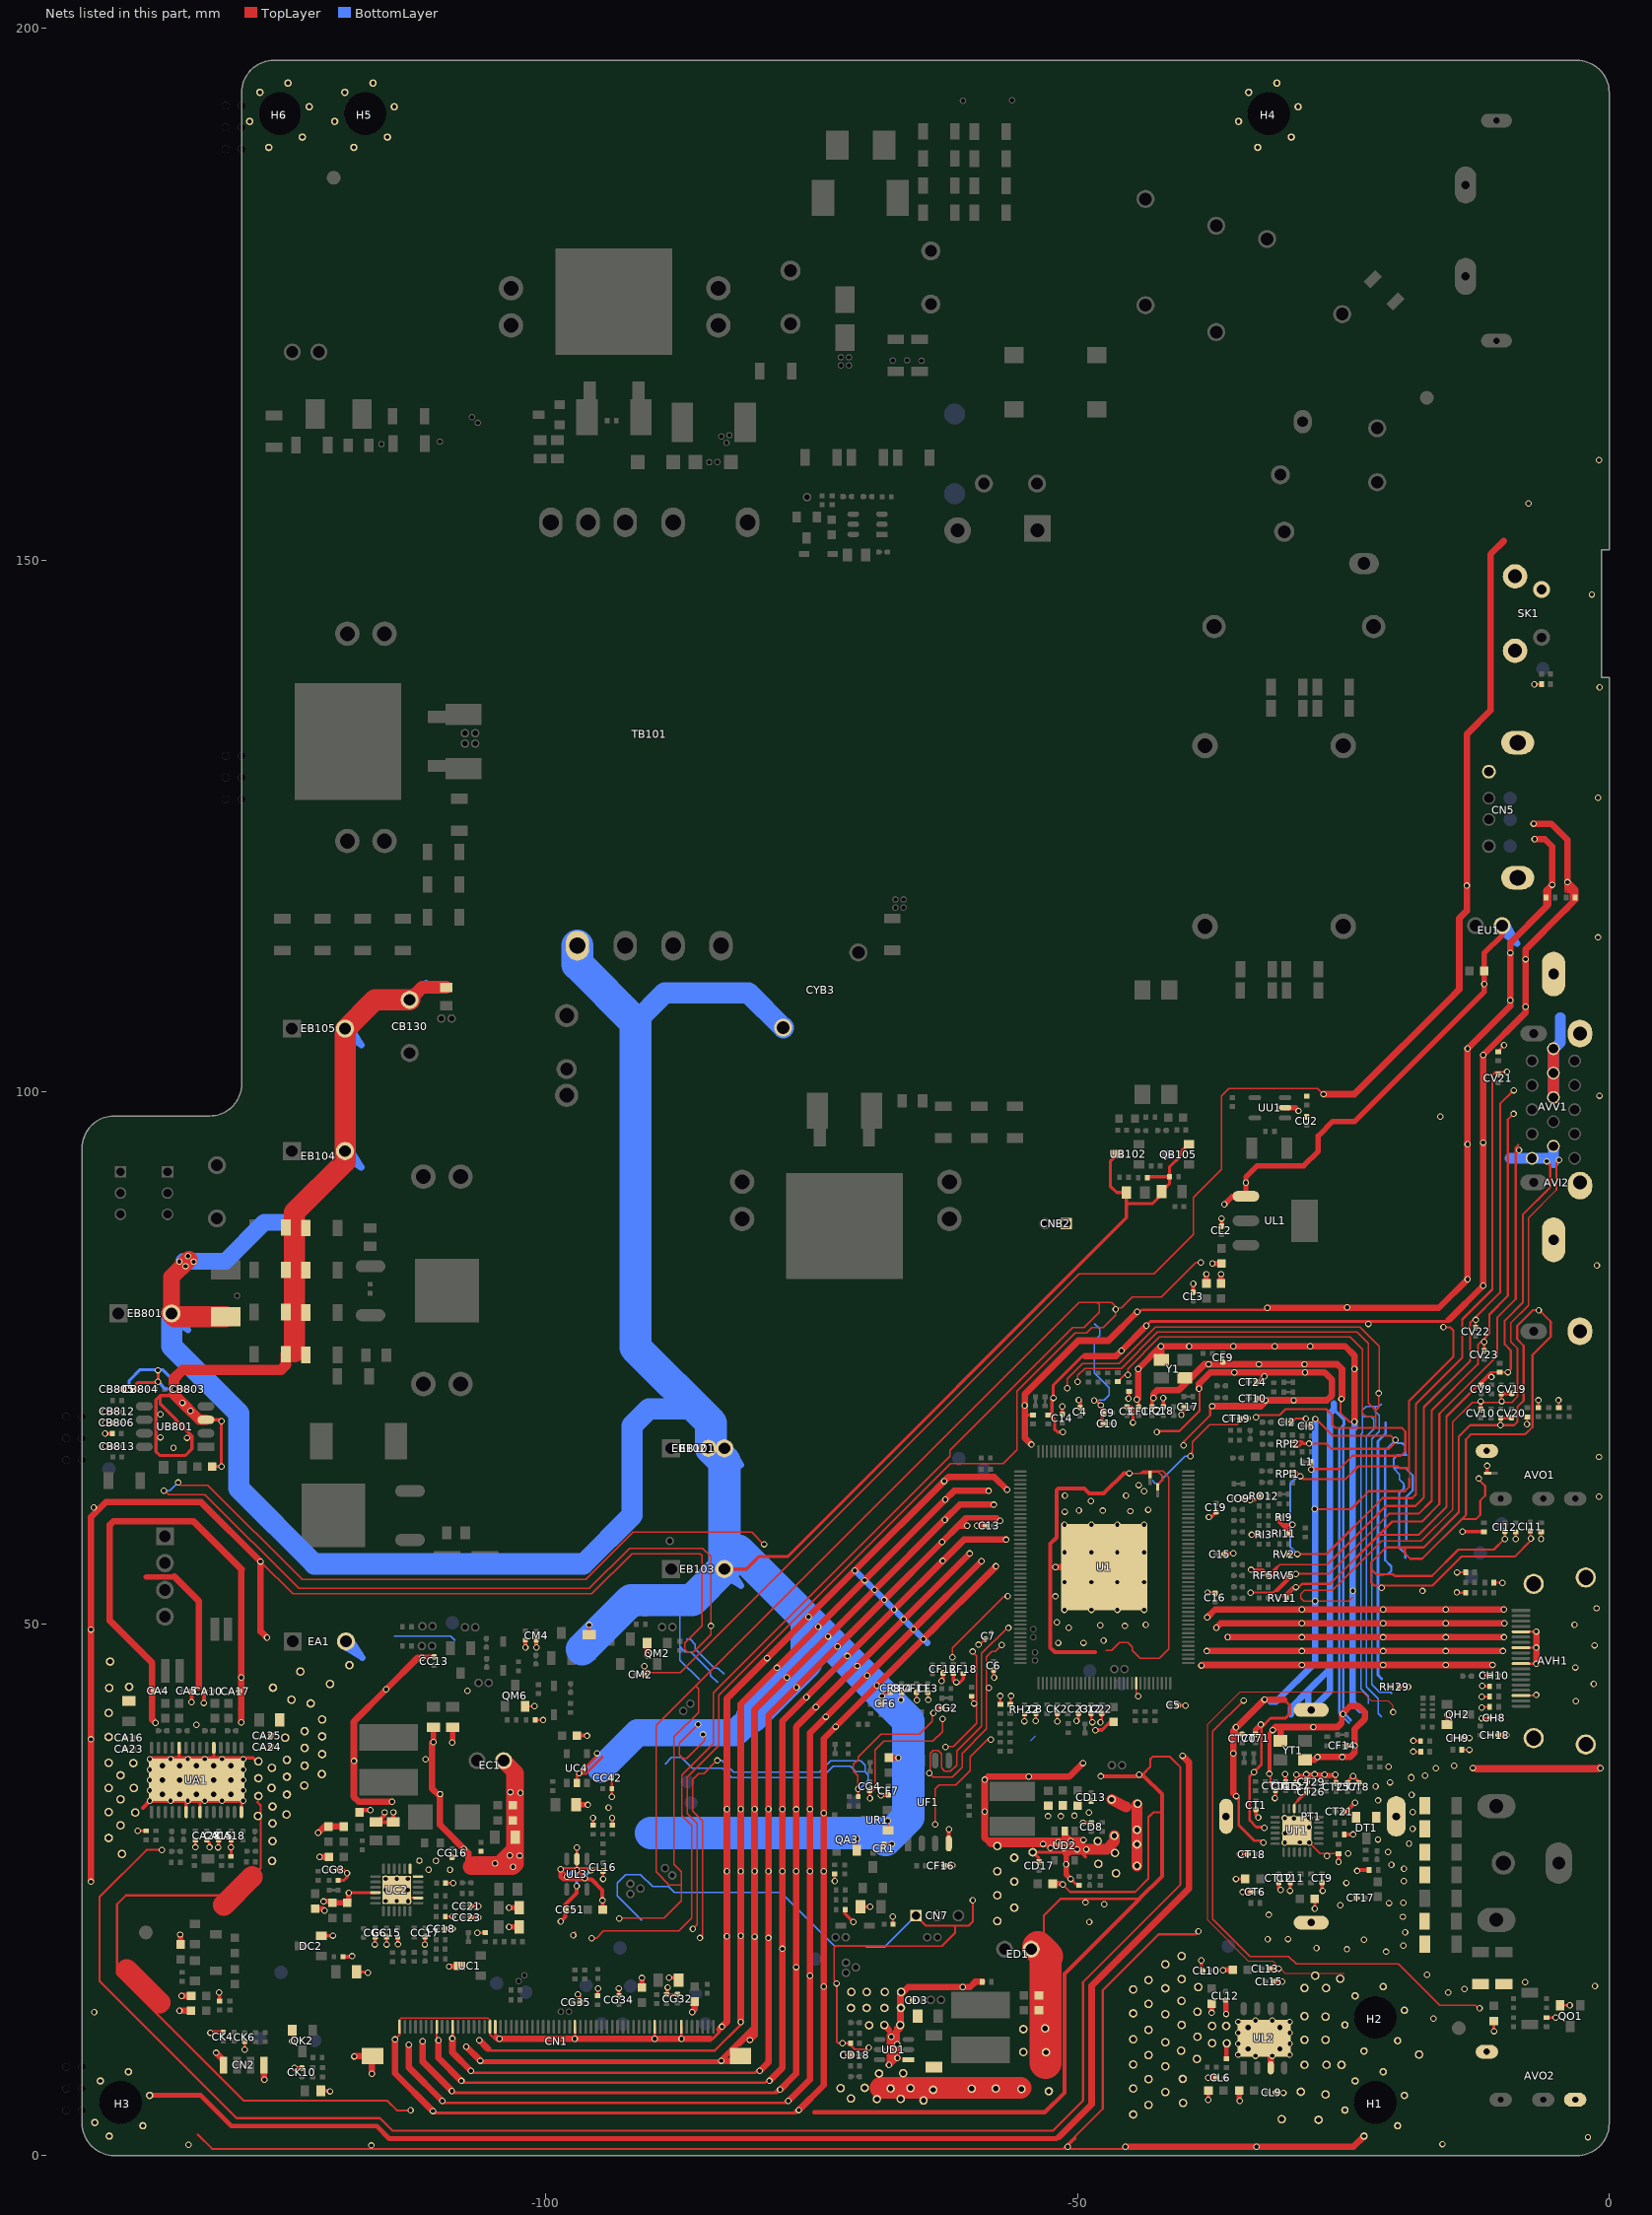
[diagram p0: the nets of this part, all layers, seen from the top]
# Altium PCB MISC86383-9.PcbDoc (part 9 of 18)
Units mm, origin at the board's own origin, x right, y up, seen from the top; angles counter-clockwise.
Board outline 143.6 x 197 mm, 2 copper layers (TopLayer, BottomLayer), stack 1.571 mm thick; 743 components, 401 nets, 2996 pads, 1077 vias.
Unrouted connection lines stored in the file: 4.

## Via types
v1: diameter 0.6, hole 0.4, TopLayer to BottomLayer, tented both sides, 993 vias
v2: diameter 0.6, hole 0.4, TopLayer to BottomLayer, 65 vias
v3: diameter 0.7, hole 0.5, TopLayer to BottomLayer, tented both sides, 15 vias
v4: diameter 0.8, hole 0.5, TopLayer to BottomLayer, tented both sides, 4 vias

## Nets (pads, with @x,y where several pads share a name; then routed paths per layer and width w, separated by ;. In a path a pad name is that pad's centre, name@x,y a point inside that pad or via, vN(x,y) a via of type N, cw(c..) or ccw(c..) an arc to the next point about the centre after c; other vN are vias at no path point) (continued)
GND: AVH1.5 AVH1.8 AVH1.11 AVH1.17 AVH1.20 AVH1.21 AVH1.22 AVH1.23 AVI2.2 AVI2.4 AVI2.6 AVO1.1 AVO2.1 AVO2.3 AVV1.5 AVV1.6 AVV1.7 AVV1.8 AVV1.10 AVV1.16 AVV1.17 C3.1 C4.1 C5.1 C6.1 C7.1 C8.1 C9.1 C10.1 C11.1 C12.1 C13.1 C14.1 C15.1 C16.1 C17.1 C18.1 C19.1 C22.1 C23.1 CA4.2@-136.92,43.698 CA4.2@-136.745,43.698 CA5.2@-133.314,43.673 CA5.2@-133.489,43.673 CA10.2@-131.982,43.66 CA10.2@-132.157,43.66 CA15.2@-130.762,29.658 CA15.2@-130.762,29.833 CA16.1 CA17.1 CA18.2@-129.594,29.658 CA18.2@-129.594,29.833 CA23.1 CA24.1 CA25.1 CA28.1 CA31.1 CA32.1 CA36.1 CB115.2 CB130.1 CB801.1 CB803.2@-133.987,72.074 CB803.2@-134.162,72.074 CB804.2@-138.5,72.06 CB804.2@-138.325,72.06 CB805.1 CB806.2@-140.77,68.885 CB806.2@-140.595,68.885 CB812.1 CB813.1 CC1.1 CC2.1 CC4.2 CC5.2 CC7.1 CC8.1 CC9.2 CC10.2 CC11.2 CC12.1 CC13.1 CC15.2@-114.98,20.53 CC15.2@-114.98,20.705 CC17.1 CC18.1 CC19.2 CC20.2 CC21.2@-107.018,23.463 CC21.2@-107.193,23.463 CC23.1 CC29.2 CC30.2 CC33.1 CC34.1 CC38.1 CC42.2@-93.783,35.496 CC42.2@-93.958,35.496 CC43.1 CC50.2 CC51.1 CD1.1 CD2.2 CD3.1 CD7.1 CD8.1 CD9.1 CD10.1 CD13.1 CD14.1 CD15.1 CD16.1 CD17.1 CD18.1 CF1.1 CF2.1 CF3.2@-64.069,43.521 CF3.2@-64.069,43.696 CF4.2@-66.548,43.517 CF4.2@-66.548,43.692 CF6.2@-68.297,42.469 CF6.2@-68.472,42.469 CF7.2@-67.783,33.871 CF7.2@-67.783,34.046 CF8.2@-67.615,43.517 CF8.2@-67.615,43.692 CF9.1 CF10.1 CF11.2@-65.151,43.517 CF11.2@-65.151,43.692 CF12.2@-62.649,45.32 CF12.2@-62.649,45.495 CF14.1 CF16.2@-62.458,27.254 CF16.2@-62.633,27.254 CG2.2@-62.582,42.05 CG2.2@-62.757,42.05 CG3.2@-119.532,26.878 CG3.2@-119.707,26.878 CG4.2@-69.545,34.297 CG4.2@-69.545,34.472 CG6.2@-116.046,20.53 CG6.2@-116.046,20.705 CG14.2 CG16.1 CG22.2 CG28.2 CG31.1 CG32.1 CG33.1 CG34.1 CG35.2@-96.743,14.402 CG35.2@-96.918,14.402 CH8.1 CH9.1 CH10.1 CH18.1 CI2.1 CI5.1 CI11.2@-7.417,58.706 CI11.2@-7.417,58.881 CI12.2@-9.804,58.83 CI12.2@-9.804,58.655 CK2.2@-51.903,41.553 CK2.2@-51.903,41.728 CK4.2@-130.333,11.424 CK4.2@-130.333,11.599 CK6.1 CK10.1 CL1.1 CL2.1 CL3.1 CL4.1 CL5.1 CL6.1 CL7.1 CL8.1 CL9.1 CL10.1 CL11.2 CL12.1 CL13.2@-31.884,17.577 CL13.2@-32.059,17.577 CL14.2 CL15.2@-31.528,16.358 CL15.2@-31.703,16.358 CL16.2@-94.615,26.689 CL16.2@-94.615,26.864 CM2.2@-90.697,45.212 CM2.2@-90.872,45.212 CM4.2@-100.902,48.444 CM4.2@-100.902,48.619 CM5.1 CN1.1 CN1.8 CN1.11 CN1.18 CN1.19 CN1.34 CN1.49 CN1.54 CN1.61 CN1.62 CN2.1 CN2.4 CN5.4 CN5.5 CN5.6 CN7.1 CNB2.1 CO9.1 CO77.2 CR1.1 CT1.1 CT2.1 CT5.1 CT6.2@-33.539,24.767 CT6.2@-33.714,24.767 CT7.1 CT8.1 CT9.2@-26.997,25.637 CT9.2@-26.997,25.812 CT10.2@-33.096,71.184 CT10.2@-33.271,71.184 CT11.1 CT12.2@-31.067,25.637 CT12.2@-31.067,25.812 CT14.1 CT15.1 CT17.2@-23.624,24.216 CT17.2@-23.799,24.216 CT18.1 CT19.1 CT21.2@-24.947,32.348 CT21.2@-25.122,32.348 CT24.1 CT25.2@-25.677,34.898 CT25.2@-25.677,35.073 CT26.1 CT27.2@-29.436,34.948 CT27.2@-29.436,35.123 CT29.1 CT41.1 CT42.1 CT43.1 CT44.1 CT45.1 CT46.1 CT47.1 CT48.1 CT70.2@-34.52,39.454 CT70.2@-34.52,39.629 CT71.1 CU1.1 CU2.2@-28.448,97.536 CU2.2@-28.448,97.711 CV9.1 CV10.1 CV19.1 CV20.1 CV21.1 CV22.1 CV23.1 CYB3.2 DB804.K DC2.3 DH2.A DH3.A DH6.A DH7.A DI1.A DI2.A DI3.A DI5.A DK1.A DK2.A DK6.A DK20.K DO1.A DO2.A DO3.A DR1.A DT1.1 DT1.3 DT2.A DT3.A DU1.A DU2.A DU3.A DU4.A DV1.A DV2.A DV3.A DV4.A DV5.A DV6.A DV7.A DV8.A EA1.2 EB101.2 EB102.2 EB103.2 EB104.2 EB105.2 EB801.2 EC1.2 ED1.2 EU1.2 H1.1 H1.2 H1.3 H1.4 H1.5 H1.6 H2.1 H2.2 H2.3 H2.4 H2.5 H2.6 H3.1 H3.2 H3.3 H3.4 H3.5 H3.6 H4.1 H4.2 H4.3 H4.4 H4.5 H4.6 H5.1 H5.2 H5.3 H5.4 H5.5 H5.6 H6.1 H6.2 H6.3 H6.4 H6.5 H6.6 L1.1 LT6.2 LT8.2 LT11.2 pad.VIA5@-17.882,9.5 pad.VIA5@-25.171,8.522 pad.VIA5@-25.298,16.612 pad.VIA5@-26.67,5.74 pad.VIA5@-26.67,10.871 pad.VIA5@-26.67,13.056 pad.VIA5@-26.568,8.534 pad.VIA5@-26.619,15.748 pad.VIA5@-27.33,3.353 pad.VIA5@-27.635,16.916 pad.VIA5@-28.651,8.534 pad.VIA5@-28.651,10.871 pad.VIA5@-28.651,13.106 pad.VIA5@-28.651,15.748 pad.VIA5@-29,5.994 pad.VIA5@-30.785,3.404 pad.VIA5@-35.966,10.54 pad.VIA5@-36.017,12.192 pad.VIA5@-37.338,10.566 pad.VIA5@-37.338,12.192 pad.VIA5@-38.71,11.176 pad.VIA5@-38.71,13.513 pad.VIA5@-38.645,15.833 pad.VIA5@-38.766,9.081 pad.VIA5@-40.073,4.944 pad.VIA5@-40.098,7.201 pad.VIA5@-40.195,16.592 pad.VIA5@-40.203,12.284 pad.VIA5@-40.208,18.748 pad.VIA5@-40.228,14.541 pad.VIA5@-40.254,9.848 pad.VIA5@-41.739,5.956 pad.VIA5@-41.739,8.392 pad.VIA5@-41.739,10.649 pad.VIA5@-41.739,13.286 pad.VIA5@-41.739,15.722 pad.VIA5@-41.739,17.979 pad.VIA5@-43.326,4.747 pad.VIA5@-43.326,7.183 pad.VIA5@-43.326,9.44 pad.VIA5@-43.326,11.813 pad.VIA5@-43.326,14.248 pad.VIA5@-43.326,16.505 pad.VIA5@-44.77,3.862 pad.VIA5@-44.77,6.298 pad.VIA5@-44.77,8.555 pad.VIA5@-44.77,10.928 pad.VIA5@-44.77,13.363 pad.VIA5@-44.77,15.62 pad.VIA5@-44.351,33.07 pad.VIA5@-44.405,27.228 pad.VIA5@-44.405,29.26 pad.VIA5@-44.405,30.632 pad.VIA5@-46.384,26.536 pad.VIA5@-46.482,28.448 pad.VIA5@-46.533,30.074 pad.VIA5@-46.787,33.477 pad.VIA5@-48.032,27.427 pad.VIA5@-48.108,29.566 pad.VIA5@-52.697,6.041 pad.VIA5@-52.967,9.703 pad.VIA5@-53.042,11.949 pad.VIA5@-54.216,28.516 pad.VIA5@-55.09,11.88 pad.VIA5@-55.103,9.738 pad.VIA5@-55.257,6.25 pad.VIA5@-55.947,23.314 pad.VIA5@-55.947,25.749 pad.VIA5@-55.947,28.006 pad.VIA5@-57.541,22.035 pad.VIA5@-57.541,24.471 pad.VIA5@-57.541,26.728 pad.VIA5@-57.541,29.101 pad.VIA5@-57.692,6.301 pad.VIA5@-59.95,6.275 pad.VIA5@-63.574,6.178 pad.VIA5@-64.478,5.173 pad.VIA5@-65.709,6.332 pad.VIA5@-66.396,7.734 pad.VIA5@-66.586,15.377 pad.VIA5@-66.608,13.875 pad.VIA5@-66.612,5.327 pad.VIA5@-66.663,12.263 pad.VIA5@-67.575,6.31 pad.VIA5@-68.15,13.875 pad.VIA5@-68.17,12.263 pad.VIA5@-68.128,15.377 pad.VIA5@-68.653,7.709 pad.VIA5@-68.869,5.301 pad.VIA5@-69.592,12.245 pad.VIA5@-69.814,15.377 pad.VIA5@-69.836,13.875 pad.VIA5@-70.01,6.361 pad.VIA5@-71.279,15.377 pad.VIA5@-71.301,13.875 pad.VIA5@-71.305,5.352 pad.VIA5@-72.268,6.335 pad.VIA5@-102.387,34.112 pad.VIA5@-102.464,28.194 pad.VIA5@-103.083,27.14 pad.VIA5@-103.327,34.163 pad.VIA5@-103.391,28.219 pad.VIA5@-104.762,27.47 pad.VIA5@-107.709,28.816 pad.VIA5@-109.004,26.86 pad.VIA5@-109.931,33.985 pad.VIA5@-110.325,27.711 pad.VIA5@-111.014,26.873 pad.VIA5@-111.887,27.724 pad.VIA5@-118.466,46.106 pad.VIA5@-120.288,44.34 pad.VIA5@-121.022,37.741 pad.VIA5@-121.022,39.41 pad.VIA5@-121.022,40.991 pad.VIA5@-121.062,35.866 pad.VIA5@-122.68,36.657 pad.VIA5@-122.68,38.326 pad.VIA5@-122.68,39.907 pad.VIA5@-122.72,34.782 pad.VIA5@-122.117,42.511 pad.VIA5@-123.084,45.51 pad.VIA5@-123.916,42.859 pad.VIA5@-124.349,33.943 pad.VIA5@-124.349,35.612 pad.VIA5@-124.349,37.192 pad.VIA5@-124.388,32.068 pad.VIA5@-124.511,39.281 pad.VIA5@-125.75,36.447 pad.VIA5@-125.654,43.993 pad.VIA5@-125.699,29.573 pad.VIA5@-125.699,31.242 pad.VIA5@-125.699,32.822 pad.VIA5@-125.739,27.698 pad.VIA5@-125.789,34.571 pad.VIA5@-127.036,33.802 pad.VIA5@-127.036,35.472 pad.VIA5@-127.036,37.052 pad.VIA5@-127.075,31.927 pad.VIA5@-133.116,84.043 pad.VIA5@-133.655,84.582 pad.VIA5@-133.871,83.617 pad.VIA5@-134.455,84.061 pad.VIA5@-138.613,32.249 pad.VIA5@-138.736,34.561 pad.VIA5@-138.789,36.901 pad.VIA5@-139.183,44.072 pad.VIA5@-139.865,28.364 pad.VIA5@-139.985,31.058 pad.VIA5@-139.985,33.494 pad.VIA5@-139.985,35.751 pad.VIA5@-140.972,46.448 pad.VIA5@-141.051,43.962 pad.VIA5@-141.108,29.858 pad.VIA5@-141.108,32.293 pad.VIA5@-141.108,34.55 pad.VIA5@-141.108,36.923 pad.VIA5@-141.108,39.359 pad.VIA5@-141.108,41.616 PT1.1 PT1.2 PT1.3 PT1.4 QA3.E QB105.E QH2.E QK2.E QM2.E QM6.E QO1.E RA1.1 RA2.JP_2K RA12.2 RA14.1 RA15.JP_2K RA18.1 RA31.1 RA38.1 RB134.1 RB140.2 RB181.1 RB183.2 RB803.1 RB818.2 RB819.2 RB820.2 RB821.2 RB837.1 RB838.1 RB839.2 RB840.1 RC3.1 RC12.1 RC18.1 RC24.1 RC27.1 RC35.2 RD5.1 RD8.2 RF5.2 RF13.2 RF18.2 RG12.1 RG13.1 RG14.1 RG16.1 RG44.1 RG58.2 RG63.2 RH22.1 RH29.2 RI3.1 RI9.1 RI10.JP_1K RI11.1 RL3.1 RL4.1 RL7.1 RM6.2 RM10.2 RO12.2 RPI1.4 RPI1.6 RPI2.4 RPI2.6 RR2.2 RU45.2 RV2.1 RV4.2 RV5.1 RV11.1 RV14.2 SK1.1 SK1.3 SK1.4 TB101.7 U1.148 U1.157 UA1.6 UA1.8 UA1.14 UA1.19 UA1.24 UA1.EPAD@-132.845,35.316 UB102.A UB801.3 UC1.3 UC2.4 UC2.14 UC2.18 UC2.19 UC2.25 UC4.2 UD1.1 UD2.2 UF1.4 UL1.1 UL2.3 UL2.EPAD UL3.2 UR1.1 UT1.10 UT1.25 UU1.2 Y1.2 Y1.4 YT1.2 YT1.4 | length 5125.2
  TopLayer w0.102: -34.178,43.614 -34.687,43.614 ; -24.93,17.145 -30.48,17.145 -31.623,18.288 -33.943,18.288 -37.776,22.121 -37.776,40.526 -34.687,43.614 ; v1(-20.312,41.681) -20.312,42.305 -20.797,42.79 -22.379,42.79 -23.203,43.614 -34.687,43.614 ; -18.772,63.663 -18.772,64.213
  TopLayer w0.127: CA31.1@-139.517,43.051 CA31.1@-139.212,42.746 ; v2(-135.903,62.522) -135.801,62.522 -135.433,62.154 -132.075,62.154 -123.235,53.315 -95.914,53.315 -92.129,57.099 -85.242,57.099 -84.468,56.325 v1(-84.468,49.797) -84.468,48.992 -86.101,47.358 -86.694,47.358 -86.936,47.6 -86.936,48.192 -85.319,49.809 -85.319,56.435 -85.475,56.591 -91.882,56.591 -95.667,52.807 -123.787,52.807 v2(-126.835,55.854) ; v2(-134.582,63.284) -134.336,63.038 -131.78,63.038 -122.89,54.148 -96.259,54.148 -91.784,58.623 -80.645,58.623 -79.502,57.48 v2(-79.477,57.48) ; CN1.1@-113.75,12.103 -113.75,12.785 -113.592,12.943 -105.475,12.943 CN1.18@-105.25,12.718 ; v1(-93.091,22.288) -93.04,22.339 -88.869,22.339 -87.273,23.936 -87.273,25.451 ; CM2.2@-90.697,45.212 -90.494,45.415 -87.326,45.415 -49.835,82.906 -42.808,82.906 -39.091,86.623 -39.091,90.077 -36.449,92.719 -36.449,99.644 -35.763,100.33 -27.407,100.33 v2(-26.873,99.797) ; -86.959,21.63 -87.486,21.103 ; v1(-86.169,21.323) -85.75,21.742 -85.75,31.24 -86.685,32.175 -86.685,35.576 -83.718,38.544 -83.718,43.289 -61.957,65.049 -57.01,65.049 -55.689,66.37 -55.689,71.877 -50.222,77.345 -49.143,77.345 -48.628,77.859 -47.561,77.859 ; -85.877,44.107 -85.648,43.878 -85.648,41.675 -87.955,39.368 -87.955,27.368 -87.273,26.685 -87.273,25.451 ; v1(-85.674,40.551) -87.447,38.778 -87.447,37.659 -87.114,37.325 -86.732,37.325 -85.065,38.993 -85.065,39.433 -85.204,39.573 v1(-85.204,39.599) ; v1(-85.509,20.46) -85.242,20.726 -85.242,31.451 -86.177,32.386 -86.177,35.366 -85.621,35.922 -85.143,35.922 -84.151,36.913 -83.861,36.913 v1(-83.861,37.143) ; -83.218,46.863 -49.855,80.226 -48.171,80.226 ; -82.852,47.229 -89.632,40.449 -89.632,26.674 -88.409,25.451 -87.273,25.451 ; v1(-72.649,16.186) -72.885,16.422 -72.885,19.571 -72.784,19.672 -62.781,19.672 -62.743,19.71 ; v1(-70.637,34.468) -70.658,34.488 -70.658,35.79 -70.688,35.79 -71.055,36.157 -71.055,36.786 -70.625,37.216 -70.625,37.505 -68.498,39.632 -64.852,39.632 -63.664,40.82 -63.664,41.543 -63.599,41.607 v1(-63.553,41.607) ; CG4.2@-69.545,34.297 -69.265,34.297 -69.03,34.532 -69.03,38.13 -68.214,38.946 -63.604,38.946 -62.686,39.864 -62.686,41.035 v1(-62.692,41.041) ; v1(-63.398,31.14) -63.398,34.468 -63.03,34.836 -61.437,34.836 -60.084,36.19 -60.084,37.503 -58.42,39.167 -58.09,39.167 -58.09,39.163 v1(-58.135,39.118) ; v1(-62.42,38.405) -62.459,38.443 -61.658,38.443 -59.474,40.627 -59.474,47.004 v1(-59.855,47.385) ; v1@-61.76,46.825 v1(-61.76,46.85) -61.76,47.736 ; -61.384,48.112 -61.76,47.736 ; -58.56,44.785 -58.56,44.199 ; v1(-58.323,43.979) -58.34,43.979 -58.56,44.199 ; v1(-57.129,48.016) -57.129,48.006 -57.737,47.398 -58.049,47.398 -58.56,46.888 -58.56,44.199 ; v1(-56.551,52.608) -56.551,52.709 -56.703,52.557 -56.939,52.557 -61.76,47.736 ; v1(-56.5,49.61) -56.5,49.56 -56.528,49.532 -56.683,49.532 -59.017,47.198 -59.017,40.366 -61.354,38.029 -61.354,36.716 -61.925,36.144 -62.484,36.144 -62.792,36.452 -62.792,37.763 -63.111,38.082 -63.579,38.082 -63.866,37.795 -63.866,36.007 v1(-63.932,35.942) -63.588,35.598 -61.753,35.598 -60.846,36.505 -60.846,37.819 -58.56,40.105 -58.56,44.199 ; v1(-50.952,72.161) -50.952,73.016 -49.504,74.464 -46.102,74.464 -42.687,77.879 -23.4,77.879 ; v1(-50,72.758) -49.974,72.733 -49.974,73.347 -49.314,74.007 -45.879,74.007 -42.464,77.422 -23.704,77.422 -22.652,76.369 -22.652,70.754 -22.247,70.349 -22.246,70.349 -21.941,70.045 ; -47.419,78.001 -47.561,77.859 ; -47.358,47.473 -46.811,47.473 -46.036,48.247 -45.252,48.247 -44.837,47.833 -44.837,47.483 -44.085,46.731 -42.286,46.731 -41.395,47.622 -41.395,63.759 -41.988,64.352 -42.411,64.352 -42.443,64.321 ; v1@-45.174,73.393 v1(-45.263,73.393) -45.263,73.977 -42.275,76.965 -24.374,76.965 -23.211,75.802 -23.211,69.803 -22.85,69.443 -21.941,69.443 ; v1(-45.109,64.152) -44.028,64.152 -43.476,64.152 RA15.JP_2K@-43.307,64.321 ; U1.148@-44.499,44.385 U1.148@-44.471,44.413 ; RA2.JP_2K@-42.456,62.855 -42.456,63.047 -42.456,63.081 -42.021,63.516 ; v1@-39.523,65.866 v1@-39.383,66.006 ; v2(-38.405,83.972) -38.862,83.972 -42.088,80.747 -44.843,80.747 -45.871,79.719 v1@-46.266,79.719 ; CT19.1@-34.66,69.27 -34.66,69.096 -35.021,68.735 -37.555,68.735 -39.19,67.099 -39.19,66.199 ; v1@-34.24,42.925 v1(-34.377,42.788) -37.281,39.885 -37.281,22.254 -33.759,18.732 -30.143,18.732 -29.407,17.996 -19.81,17.996 -15.938,14.124 -12.6,14.124 -12.192,13.716 v1(-12.192,13.843) ; -31.275,55.273 -30.977,55.571 -26.507,55.571 -26.426,55.652 ; v1@-24.089,30.177 v1(-24.076,30.19) ; -23.374,77.854 -21.625,76.104 -21.625,71.539 v1@-21.658,71.572 ; -22.081,68.415 -21.941,68.555 -21.941,69.443 ; v1(-21.658,71.669) v1@-21.658,71.572 ; v1@-18.529,31.013 -18.529,30.759 v1(-18.491,30.721) ; -4.148,119.108 -4.148,118.841 -4.08,118.773 -3.745,118.773 -3.634,118.661 -3.634,117.953 ; -4.105,117.192 -4.097,117.184 ; -3.864,117.6 -3.634,117.83 -3.634,117.953 ; -3.745,117.842 -3.634,117.953 ; v1@-95.567,20.422 v1(-95.694,20.422) -95.631,20.358 v1@-95.567,20.422 ; v1@-95.567,20.422 -95.245,20.422 -94.564,21.103 -87.486,21.103 ; -87.486,21.103 -86.258,22.33 -86.258,31.03 -87.193,31.965 -87.193,35.787 -84.226,38.754 -84.226,43.499 -61.971,65.754 -61.971,66.314 -50.432,77.853 -49.39,77.853 -47.963,79.28 -47.963,80.017 -48.171,80.226 ; -48.171,80.226 -46.773,80.226 v1@-46.266,79.719 ; -47.561,77.859 -46.406,79.015 v1(-46.406,79.579) v1@-46.266,79.719 ; v1@-39.383,66.006 -39.19,66.199 ; v1@-39.383,66.006 v1(-39.383,65.761) -39.19,65.953 -39.19,66.199 ; -21.941,69.443 -21.941,70.045 ; -21.941,70.045 -21.658,70.327 v1@-21.658,71.572
  TopLayer w0.152: UT1.25@-29.36,30.57 v1(-28.21,29.42) -27.182,28.393 LT6.2@-25.435,28.393 ; -24.137,52.5 -24.503,52.133 v1(-27.661,52.133) -28.727,52.133 -29.002,52.408 -29.002,52.797 -28.639,53.16 -26.016,53.16 -21.403,57.772 -19.461,57.772 -17.681,57.773 -14.719,60.735 -14.719,68.974 -12.874,70.819 v1@-12.09,70.819 ; v1(-12.09,70.917) v1@-12.09,70.819 ; v1@-12.084,70.813 v1@-12.09,70.819 ; v1@-11.074,73.101 v1(-11.074,73.203) ; v1(-10.109,70.917) -10.109,71.069 v1@-10.102,71.076 ; v1(-7.738,68.779) -7.738,68.922 -7.717,68.943 DI1.A@-7.717,69.457 ; v1(-4.699,93.599) -4.966,93.332 -4.966,90.801 -7.595,88.172 -7.595,79.943 -9.237,78.301 -9.237,76.513 -8.631,75.907 -8.631,71.353 -9.166,70.819 -12.084,70.819 v1@-12.09,70.819
  TopLayer w0.178: U1.148@-44.471,44.413 -44.471,43.446 v1@-44.223,43.199 ; v1(-44.29,43.199) v1@-44.223,43.199 ; v1@-44.199,43.174 v1@-44.223,43.199 ; RPI1.4@-29.797,64.349 -29.75,64.302 -29.397,64.302 -29.074,63.98 v1@-29.074,63.849
  TopLayer w0.191: UT1.25@-29.61,30.82 UT1.25@-29.36,30.57 ; UT1.10@-29.61,32.62 -29.61,33.038 -29.252,33.397